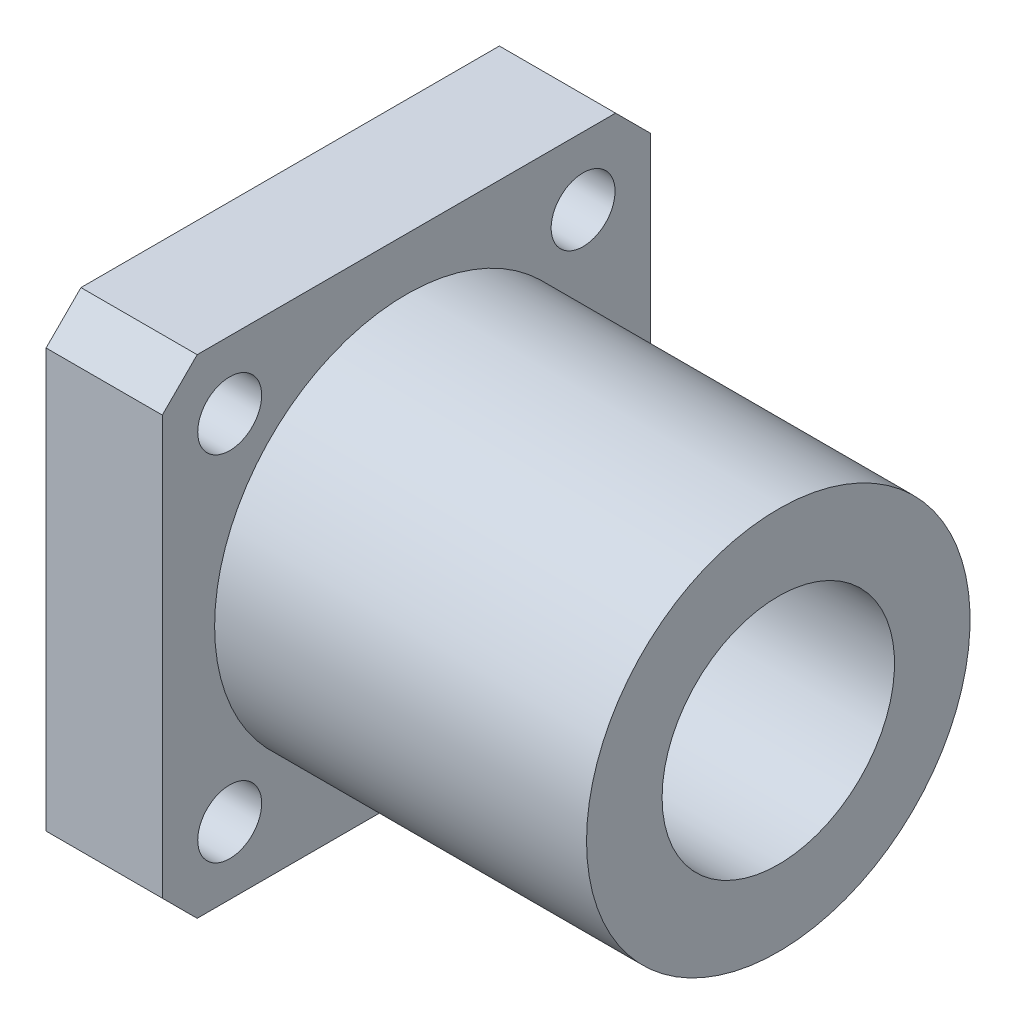
from build123d import *

# Parameters (mm, degrees)
SKETCH1_W                  = 42
SKETCH1_H                  = 42
BOSS_EXTRUDE1_DEPTH        = 10
SKETCH2_R                  = 16.5
BOSS_EXTRUDE2_DEPTH        = 32
F_5_5_5_5_DIAMETER_HOLE1_D = 5.5
SKETCH7_R                  = 10
CUT_EXTRUDE1_DEPTH         = 52.439284598
CHAMFER1_SIZE              = 3


with BuildPart() as part:
    # Sketch1 → Boss-Extrude1 (new body)
    with BuildSketch(Plane(origin=(0, 0, 0), x_dir=(0, 0, -1), z_dir=(1, 0, 0))):
        Rectangle(SKETCH1_W, SKETCH1_H)
    extrude(amount=BOSS_EXTRUDE1_DEPTH)

    # Sketch2 → Boss-Extrude2 (add)
    with BuildSketch(Plane(origin=(10, 0, 0), x_dir=(0, 0, -1), z_dir=(1, 0, 0))):
        with Locations(Location((0, 0, 0), (0, 0, 180))):
            Circle(SKETCH2_R)
    extrude(amount=BOSS_EXTRUDE2_DEPTH)

    # Ø5.5 (5.5) Diameter Hole1 (through all)
    with Locations(Plane.ZY):
        with Locations((-15.202795796, 15.202795796), (15.202795796, 15.202795796), (15.202795796, -15.202795796), (-15.202795796, -15.202795796)):
            Hole(F_5_5_5_5_DIAMETER_HOLE1_D / 2)

    # Sketch7 → Cut-Extrude1 (cut, through all)
    with BuildSketch(Plane.ZY):
        Circle(SKETCH7_R)
    extrude(amount=-CUT_EXTRUDE1_DEPTH, mode=Mode.SUBTRACT)

    # Chamfer1
    chamfer1_edges = [part.edges().sort_by_distance(p)[0] for p in [
        (5, 21, -21),
        (5, -21, -21),
        (5, -21, 21),
        (5, 21, 21),
    ]]
    chamfer(chamfer1_edges, length=CHAMFER1_SIZE)


solid = part.part
